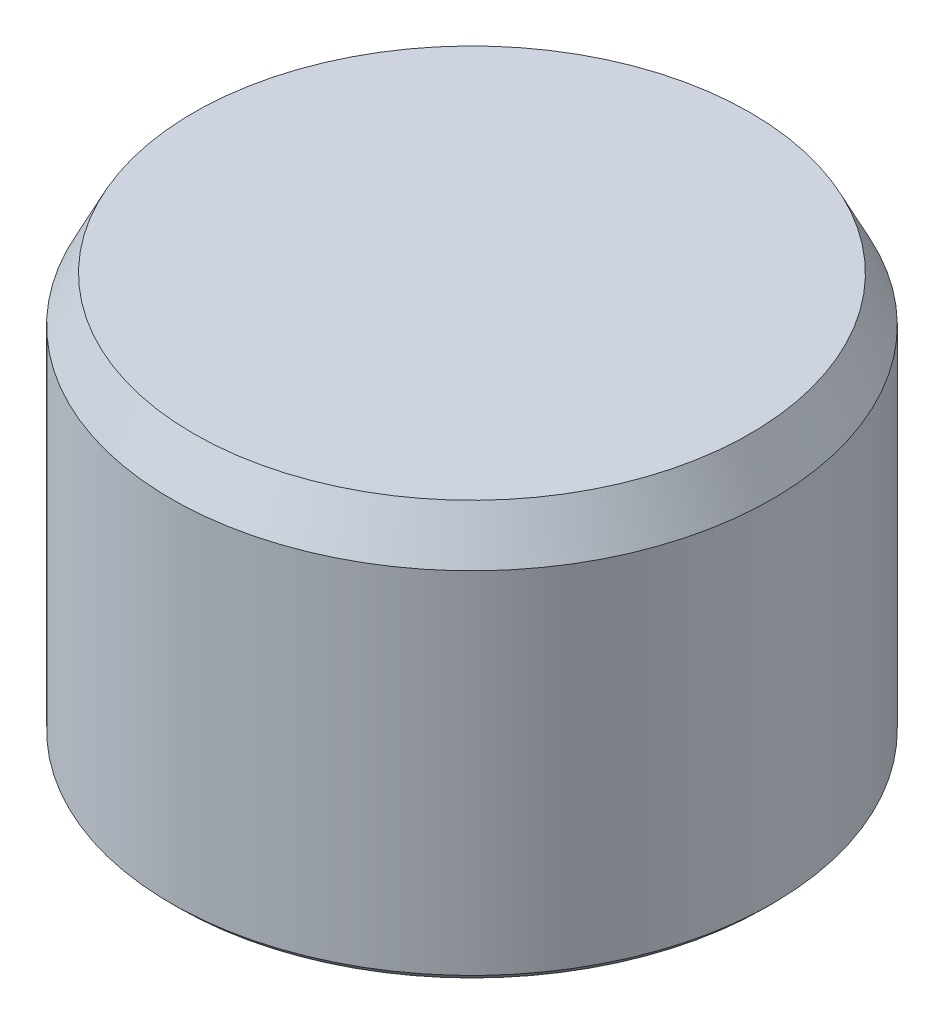
from build123d import *

# Parameters (mm, degrees)
SKETCH1_W      = 20
SKETCH1_H      = 26.8
CHAMFER1_SIZE  = 1.5
CHAMFER1_SIZE2 = 3
CHAMFER2_SIZE  = 0.5


with BuildPart() as part:
    # Sketch1 → Revolve1 (revolve)
    with BuildSketch(Plane.XY, mode=Mode.PRIVATE) as revolve1_sk:
        with Locations((10, 0)):
            Rectangle(SKETCH1_W, SKETCH1_H)
    revolve(revolve1_sk.sketch.rotate(Axis((0, 0, 0), (0, 1, 0)), 90), axis=Axis((0, 0, 0), (0, 1, 0)))

    # Chamfer1
    chamfer1_edges = [part.edges().sort_by_distance(p)[0] for p in [
        (0, 13.4, 20),
    ]]
    chamfer1_side = [part.faces().sort_by_distance(p)[0] for p in [
        (0, 13.4, 0),
    ]]
    chamfer(chamfer1_edges, length=CHAMFER1_SIZE, length2=CHAMFER1_SIZE2, reference=chamfer1_side[0])

    # Chamfer2
    chamfer2_edges = [part.edges().sort_by_distance(p)[0] for p in [
        (0, -13.4, 20),
    ]]
    chamfer(chamfer2_edges, length=CHAMFER2_SIZE)


solid = part.part
